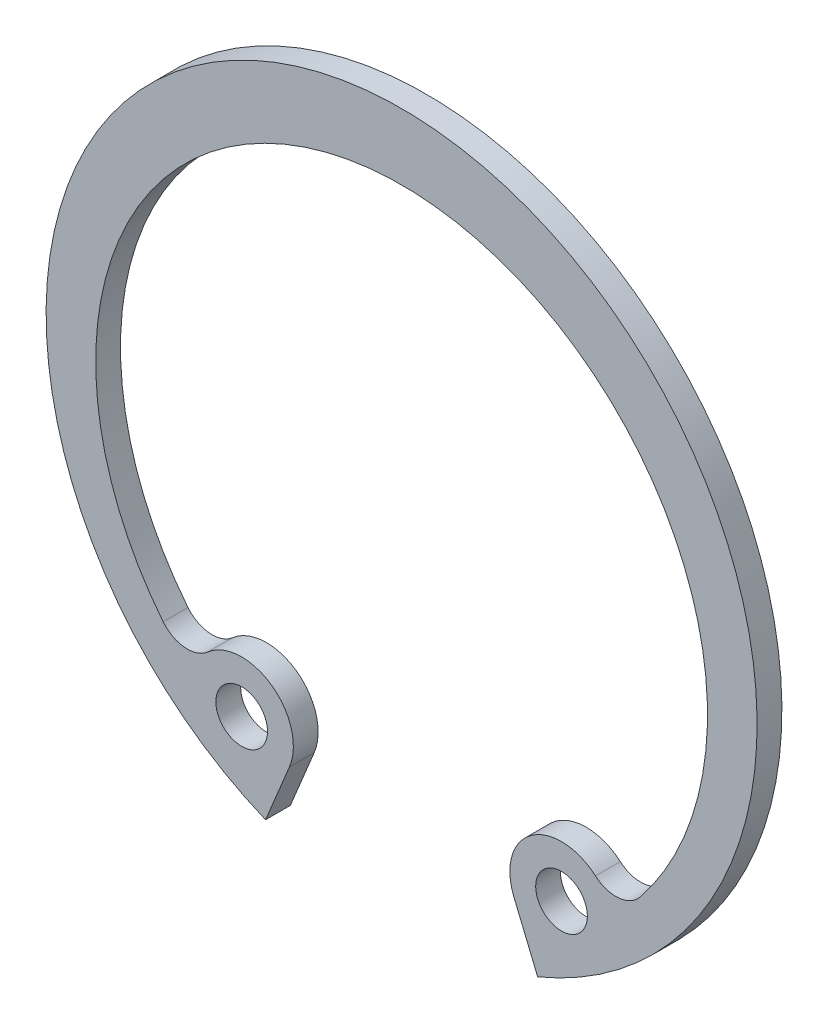
from build123d import *

# Parameters (mm, degrees)
SKETCH_1_R      = 1.25
EXTRUDE_1_DEPTH = 1.2


with BuildPart() as part:
    # 草图1 → 凸台-拉伸1 (new body)
    with BuildSketch(Plane.XY):
        with BuildLine():
            Line((5.426958413, -13.101836603), (6.582155037, -15.890727959))
            ThreePointArc((6.582155037, -15.890727959), (0, 17.2), (-6.582155037, -15.890727959))
            Line((-6.582155037, -15.890727959), (-5.426958413, -13.101836603))
            ThreePointArc((-5.426958413, -13.101836603), (-6.278083953, -10.114718223), (-9.380614428, -10.261672481))
            ThreePointArc((-9.380614428, -10.261672481), (-10.498981278, -10.625780527), (-11.536197995, -10.071253196))
            ThreePointArc((-11.536197995, -10.071253196), (0, 14), (11.536197995, -10.071253196))
            ThreePointArc((11.536197995, -10.071253196), (10.498981278, -10.625780527), (9.380614428, -10.261672481))
            ThreePointArc((9.380614428, -10.261672481), (6.278083953, -10.114718223), (5.426958413, -13.101836603))
        make_face()
        with Locations(Location((-7.736657244, -12.145128022, 0), (0, 0, 180))):
            Circle(SKETCH_1_R, mode=Mode.SUBTRACT)
        with Locations(Location((7.736657244, -12.145128022, 0), (0, 0, 180))):
            Circle(SKETCH_1_R, mode=Mode.SUBTRACT)
    extrude(amount=-EXTRUDE_1_DEPTH)


solid = part.part
